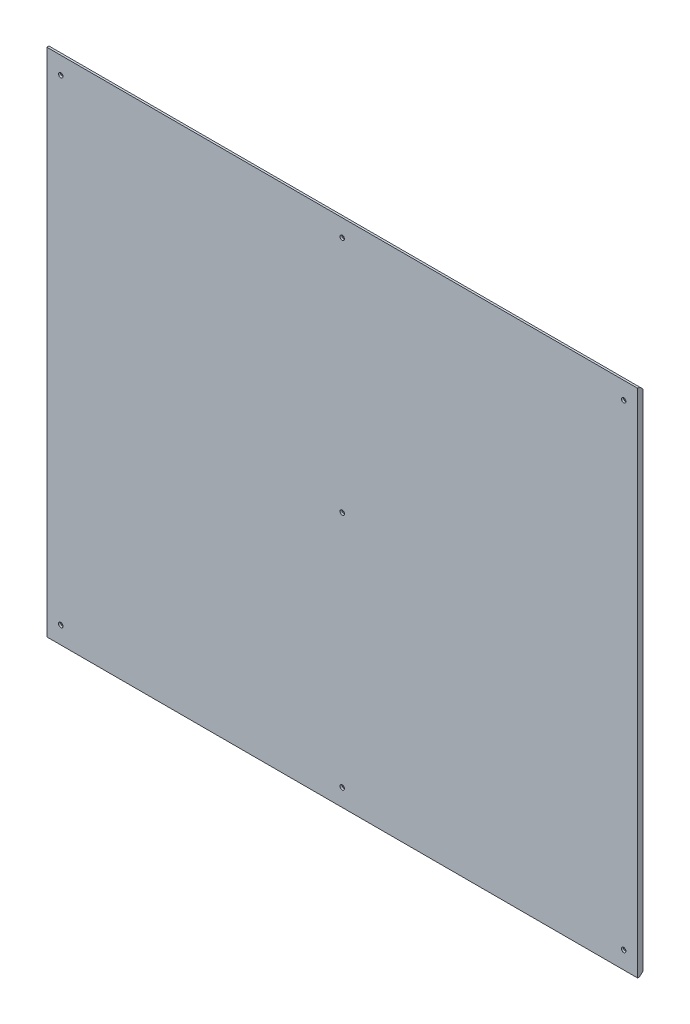
SolidWorks part; units mm, degrees
ref_plane "前视基准面" through (0, 0, 0) normal (0, 0, 1) x (1, 0, 0)
ref_plane "上视基准面" through (0, 0, 0) normal (0, 1, 0) x (1, 0, 0)
ref_plane "右视基准面" through (0, 0, 0) normal (1, 0, 0) x (0, 0, -1)
sketch "草图1" plane through (0, 0, 0) normal (0, 0, 1) x (1, 0, 0)
  line L1 (-425, 367.5) -> (425, 367.5)
  line L2 (-425, 367.5) -> (-425, -367.5)
  line L3 (-425, -367.5) -> (425, -367.5)
  line L4 (425, 367.5) -> (425, -367.5)
  line L5 (-425, 367.5) -> (425, -367.5) construction
  line L6 (-425, -367.5) -> (425, 367.5) construction
  point P0 (0, 0)
  dimension "D1" = 850
  dimension "D2" = 735
extrude "凸台-拉伸1" add sketch "草图1" along normal blind 8
chamfer "倒角1" distance 5 angle 45 2 edges at (0, 367.5, 0) (0, -367.5, 0)
sketch "草图2" plane through (0, 0, 0) normal (0, 0, -1) x (-1, 0, 0)
  line L3 (-425, -362.5) -> (-425, 362.5) construction
  line L4 (-425, 367.5) -> (425, 367.5) construction
  circle A0 centre (-405, 342.5) radius 8.25
  circle A1 centre (0, 342.5) radius 8.25
  circle A2 centre (405, 342.5) radius 8.25
  circle A3 centre (-405, -342.5) radius 8.25
  circle A4 centre (0, -342.5) radius 8.25
  circle A5 centre (405, -342.5) radius 8.25
  dimension "D1" = 16.5
  dimension "D2" = 405
  dimension "D3" = 405
  dimension "D4" = 685
  dimension "D5" = 25
  dimension "D6" = 20
extrude "切除-拉伸1" cut sketch "草图2" against normal blind 5 draft 45
sketch "草图3" plane through (0, 0, 8) normal (0, 0, 1) x (1, 0, 0)
  line L0 (-425, 367.5) -> (-425, -367.5) construction
  line L1 (425, 367.5) -> (-425, 367.5) construction
  circle A0 centre (-405, 342.5) radius 3.25
  circle A1 centre (0, 342.5) radius 3.25
  circle A2 centre (405, 342.5) radius 3.25
  circle A3 centre (-405, -342.5) radius 3.25
  circle A4 centre (0, -342.5) radius 3.25
  circle A5 centre (405, -342.5) radius 3.25
  dimension "D1" = 6.5
  dimension "D2" = 405
  dimension "D3" = 810
  dimension "D4" = 20
  dimension "D5" = 685
  dimension "D6" = 25
extrude "切除-拉伸2" cut sketch "草图3" against normal blind 3
sketch "草图4" plane through (0, 0, 0) normal (0, 0, -1) x (-1, 0, 0)
  circle A0 centre (0, 0) radius 8.25
  dimension "D1" = 16.5
extrude "切除-拉伸3" cut sketch "草图4" against normal blind 5 draft 45
sketch "草图5" plane through (0, 0, 5) normal (0, 0, -1) x (-1, 0, 0)
  circle A1 centre (0, 0) radius 3.25
  circle A2 centre (0, 0) radius 3.25
  dimension "D1" = 0
extrude "切除-拉伸4" cut sketch "草图5" against normal blind 5
